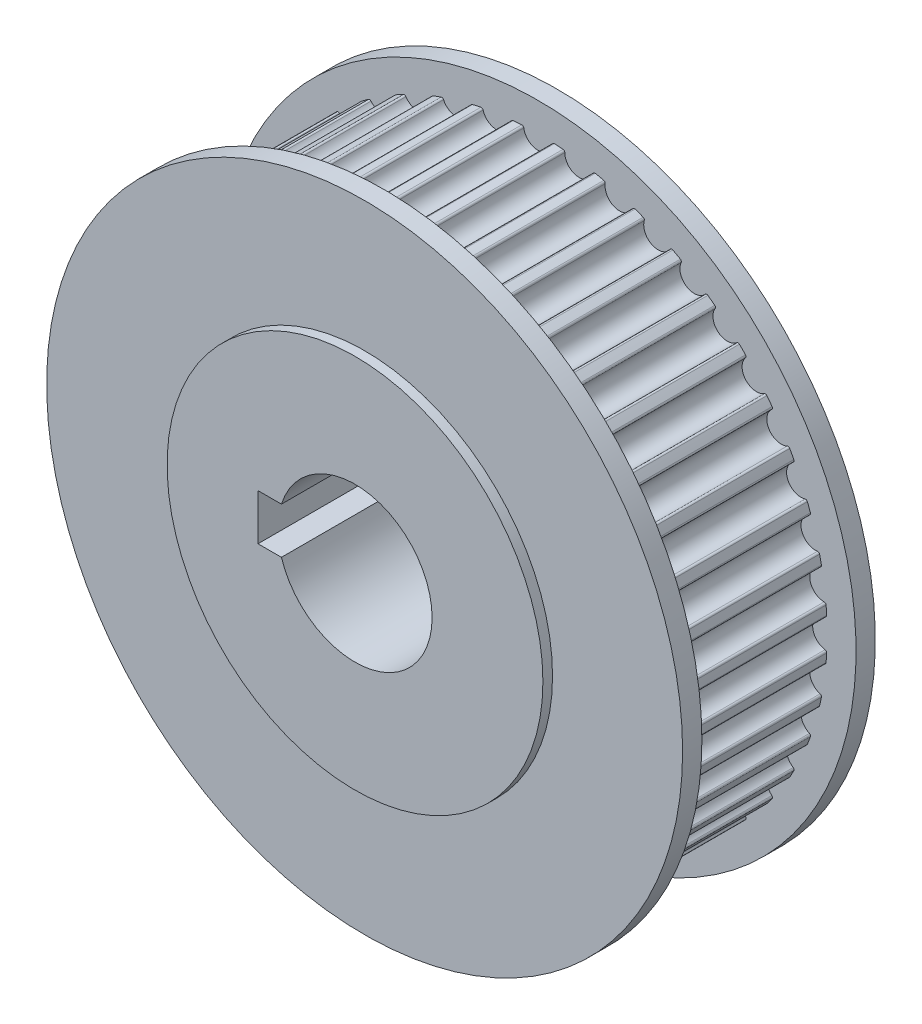
from build123d import *

# Parameters (mm, degrees)
SKETCH1_R                = 30
BOSS_EXTRUDE1_DEPTH      = 16
SKETCH2_R                = 1.5
CUT_EXTRUDE1_DEPTH       = 16
FILLET1_R                = 0.2
CIRPATTERN1_COUNT        = 44
FILLET1_OF_CIRPATTERN1_R = 0.2
SKETCH3_R                = 33
BOSS_EXTRUDE2_DEPTH      = 2
BOSS_EXTRUDE3_START      = 2
SKETCH4_R                = 33
BOSS_EXTRUDE3_DEPTH      = 2
SKETCH5_R                = 19.5
BOSS_EXTRUDE4_DEPTH      = 1
BOSS_EXTRUDE5_START      = 1
SKETCH6_R                = 19.5
BOSS_EXTRUDE5_DEPTH      = 1
CUT_EXTRUDE2_REACH       = 53.595


with BuildPart() as part:
    # Sketch1 → Boss-Extrude1 (new body)
    with BuildSketch(Plane.XY):
        Circle(SKETCH1_R)
    extrude(amount=BOSS_EXTRUDE1_DEPTH)

    # Sketch2 → Cut-Extrude1 (cut)
    with BuildSketch(Plane.XY.offset(16)):
        with Locations((0, 30)):
            Circle(SKETCH2_R)
    cut_extrude1 = extrude(amount=-CUT_EXTRUDE1_DEPTH, mode=Mode.SUBTRACT)

    # Fillet1
    fillet1_edges = [part.edges().sort_by_distance(p)[0] for p in [
        (1.499531177, 29.9625, 8),
        (-1.499531177, 29.9625, 8),
    ]]
    fillet(fillet1_edges, radius=FILLET1_R)

    # CirPattern1: Cut-Extrude1 ×44 about axis
    cirpattern1_axis = Axis((0, 0, 0), (0, 0, 1))
    for i in range(1, CIRPATTERN1_COUNT):
        add(cut_extrude1.rotate(cirpattern1_axis, i * 360 / CIRPATTERN1_COUNT), mode=Mode.SUBTRACT)

    # Fillet1 of CirPattern1
    fillet1_of_cirpattern1_edges = [part.edges().sort_by_distance(p)[0] for p in [
        (-2.77984023, 29.870930489, 8),
        (-5.748376453, 29.444119415, 8),
        (-7.002622107, 29.171274974, 8),
        (-9.880201362, 28.326341469, 8),
        (-11.082850791, 27.877776424, 8),
        (-13.810893863, 26.631920898, 8),
        (-14.937464593, 26.016766739, 8),
        (-17.460436393, 24.395351216, 8),
        (-18.487994692, 23.626130709, 8),
        (-20.754534789, 21.662162535, 8),
        (-21.662162535, 20.754534789, 8),
        (-23.626130709, 18.487994692, 8),
        (-24.395351216, 17.460436393, 8),
        (-26.016766739, 14.937464593, 8),
        (-26.631920898, 13.810893863, 8),
        (-27.877776424, 11.082850791, 8),
        (-28.326341469, 9.880201362, 8),
        (-29.171274974, 7.002622107, 8),
        (-29.444119415, 5.748376453, 8),
        (-29.870930489, 2.77984023, 8),
        (-29.9625, 1.499531177, 8),
        (-29.9625, -1.499531177, 8),
        (-29.870930489, -2.77984023, 8),
        (-29.444119415, -5.748376453, 8),
        (-29.171274974, -7.002622107, 8),
        (-28.326341469, -9.880201362, 8),
        (-27.877776424, -11.082850791, 8),
        (-26.631920898, -13.810893863, 8),
        (-26.016766739, -14.937464593, 8),
        (-24.395351216, -17.460436393, 8),
        (-23.626130709, -18.487994692, 8),
        (-21.662162535, -20.754534789, 8),
        (-20.754534789, -21.662162535, 8),
        (-18.487994692, -23.626130709, 8),
        (-17.460436393, -24.395351216, 8),
        (-14.937464593, -26.016766739, 8),
        (-13.810893863, -26.631920898, 8),
        (-11.082850791, -27.877776424, 8),
        (-9.880201362, -28.326341469, 8),
        (-7.002622107, -29.171274974, 8),
        (-5.748376453, -29.444119415, 8),
        (-2.77984023, -29.870930489, 8),
        (-1.499531177, -29.9625, 8),
        (1.499531177, -29.9625, 8),
        (2.77984023, -29.870930489, 8),
        (5.748376453, -29.444119415, 8),
        (7.002622107, -29.171274974, 8),
        (9.880201362, -28.326341469, 8),
        (11.082850791, -27.877776424, 8),
        (13.810893863, -26.631920898, 8),
        (14.937464593, -26.016766739, 8),
        (17.460436393, -24.395351216, 8),
        (18.487994692, -23.626130709, 8),
        (20.754534789, -21.662162535, 8),
        (21.662162535, -20.754534789, 8),
        (23.626130709, -18.487994692, 8),
        (24.395351216, -17.460436393, 8),
        (26.016766739, -14.937464593, 8),
        (26.631920898, -13.810893863, 8),
        (27.877776424, -11.082850791, 8),
        (28.326341469, -9.880201362, 8),
        (29.171274974, -7.002622107, 8),
        (29.444119415, -5.748376453, 8),
        (29.870930489, -2.77984023, 8),
        (29.9625, -1.499531177, 8),
        (29.9625, 1.499531177, 8),
        (29.870930489, 2.77984023, 8),
        (29.444119415, 5.748376453, 8),
        (29.171274974, 7.002622107, 8),
        (28.326341469, 9.880201362, 8),
        (27.877776424, 11.082850791, 8),
        (26.631920898, 13.810893863, 8),
        (26.016766739, 14.937464593, 8),
        (24.395351216, 17.460436393, 8),
        (23.626130709, 18.487994692, 8),
        (21.662162535, 20.754534789, 8),
        (20.754534789, 21.662162535, 8),
        (18.487994692, 23.626130709, 8),
        (17.460436393, 24.395351216, 8),
        (14.937464593, 26.016766739, 8),
        (13.810893863, 26.631920898, 8),
        (11.082850791, 27.877776424, 8),
        (9.880201362, 28.326341469, 8),
        (7.002622107, 29.171274974, 8),
        (5.748376453, 29.444119415, 8),
        (2.77984023, 29.870930489, 8),
    ]]
    fillet(fillet1_of_cirpattern1_edges, radius=FILLET1_OF_CIRPATTERN1_R)

    # Sketch3 → Boss-Extrude2 (add)
    with BuildSketch(Plane.XY.offset(16)):
        Circle(SKETCH3_R)
    extrude(amount=BOSS_EXTRUDE2_DEPTH)

    # Sketch4 → Boss-Extrude3 (add)
    with BuildSketch(Plane(origin=(0, 0, 0), x_dir=(-1, 0, 0), z_dir=(0, 0, -1)).offset(BOSS_EXTRUDE3_START)):
        with Locations(Location((0, 0, 0), (0, 0, 180))):
            Circle(SKETCH4_R)
    extrude(amount=-BOSS_EXTRUDE3_DEPTH)

    # Sketch5 → Boss-Extrude4 (add)
    with BuildSketch(Plane.XY.offset(18)):
        Circle(SKETCH5_R)
    extrude(amount=BOSS_EXTRUDE4_DEPTH)

    # Sketch6 → Boss-Extrude5 (add)
    with BuildSketch(Plane(origin=(0, 0, -2), x_dir=(-1, 0, 0), z_dir=(0, 0, -1)).offset(BOSS_EXTRUDE5_START)):
        with Locations(Location((0, 0, 0), (0, 0, 180))):
            Circle(SKETCH6_R)
    extrude(amount=-BOSS_EXTRUDE5_DEPTH)

    # Sketch7 → Cut-Extrude2 (cut, up to next)
    with BuildSketch(Plane(origin=(0, 0, -3), x_dir=(-1, 0, 0), z_dir=(0, 0, -1)), mode=Mode.PRIVATE) as cut_extrude2_sk1:
        with BuildLine():
            Line((10.067351233, 2.388297135), (7.635184136, 2.388297135))
            ThreePointArc((7.635184136, 2.388297135), (-8, 0), (7.635184136, -2.388297135))
            Line((7.635184136, -2.388297135), (10.067351233, -2.388297135))
            Line((10.067351233, -2.388297135), (10.067351233, 2.388297135))
        make_face()
    cut_extrude2_tool1 = extrude(cut_extrude2_sk1.sketch, amount=-CUT_EXTRUDE2_REACH, mode=Mode.PRIVATE) & part.part
    add(cut_extrude2_tool1.solids().sort_by_distance((-0.443225, 0, -3))[0], mode=Mode.SUBTRACT)


solid = part.part
